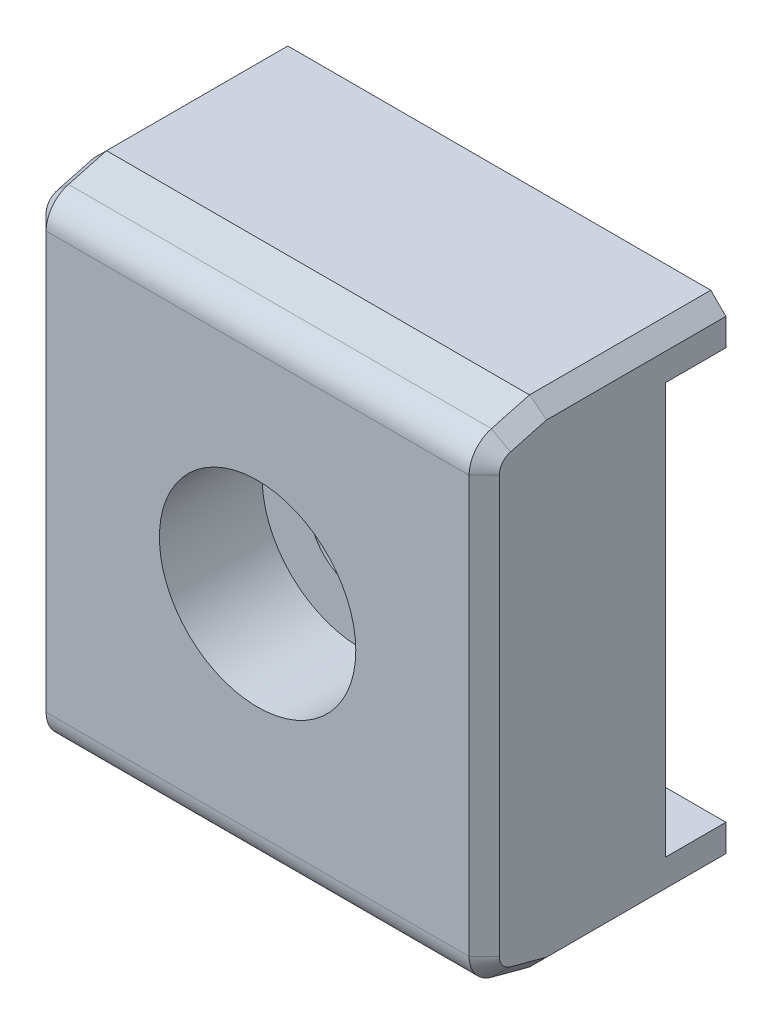
from build123d import *

# Parameters (mm, degrees)
EXTRUDE_1_DEPTH              = 15
CHAMFER_1_SIZE               = 0.5
HOLE_WIZARD_M3_1_D           = 3.4
HOLE_WIZARD_M3_1_DEPTH       = 10
HOLE_WIZARD_M3_1_CBORE_D     = 6.5
HOLE_WIZARD_M3_1_CBORE_DEPTH = 3.4
HOLE_WIZARD_M3_1_TIP         = 1.021463052


with BuildPart() as part:
    # 草图2 → 凸台-拉伸1 (new body)
    with BuildSketch(Plane.ZY.offset(7.5)):
        with BuildLine():
            Line((-6, -6.8), (-8, -6.8))
            Line((-8, -6.8), (-8, -8.2))
            Line((-8, -8.2), (-2, -8.2))
            Line((-2, -8.2), (-0.741180955, -7.862700453))
            ThreePointArc((-0.741180955, -7.862700453), (-0.20664666, -7.505536056), (0, -6.896774627))
            Line((0, -6.896774627), (0, 6.896774627))
            ThreePointArc((0, 6.896774627), (-0.20664666, 7.505536056), (-0.741180955, 7.862700453))
            Line((-0.741180955, 7.862700453), (-2, 8.2))
            Line((-2, 8.2), (-8, 8.2))
            Line((-8, 8.2), (-8, 7.7))
            Line((-8, 7.7), (-8, 6.8))
            Line((-8, 6.8), (-6, 6.8))
            Line((-6, 6.8), (-6, -6.8))
        make_face()
    extrude(amount=-EXTRUDE_1_DEPTH)

    # 倒角1
    chamfer_1_edges = [part.edges().sort_by_distance(p)[0] for p in [
        (-7.5, 8.2, -5),
        (-7.5, 8.031350227, -1.370590477),
        (-7.5, 7.505536056, -0.20664666),
        (-7.5, 0, 0),
        (-7.5, -7.505536056, -0.20664666),
        (-7.5, -8.031350227, -1.370590477),
        (-7.5, -8.2, -5),
        (7.5, -8.2, -5),
        (7.5, -8.031350227, -1.370590477),
        (7.5, -7.505536056, -0.20664666),
        (7.5, 0, 0),
        (7.5, 7.505536056, -0.20664666),
        (7.5, 8.031350227, -1.370590477),
        (7.5, 8.2, -5),
    ]]
    chamfer(chamfer_1_edges, length=CHAMFER_1_SIZE)

    # M3 六角凹头螺钉的柱形沉头孔1
    with Locations(Plane.XY):
        with Locations((0, 0)):
            CounterBoreHole(HOLE_WIZARD_M3_1_D / 2, HOLE_WIZARD_M3_1_CBORE_D / 2, HOLE_WIZARD_M3_1_CBORE_DEPTH, depth=HOLE_WIZARD_M3_1_DEPTH)
            with Locations((0, 0, -(HOLE_WIZARD_M3_1_DEPTH + HOLE_WIZARD_M3_1_TIP / 2))):  # 118° drill point
                Cone(0, HOLE_WIZARD_M3_1_D / 2, HOLE_WIZARD_M3_1_TIP, mode=Mode.SUBTRACT)


solid = part.part
